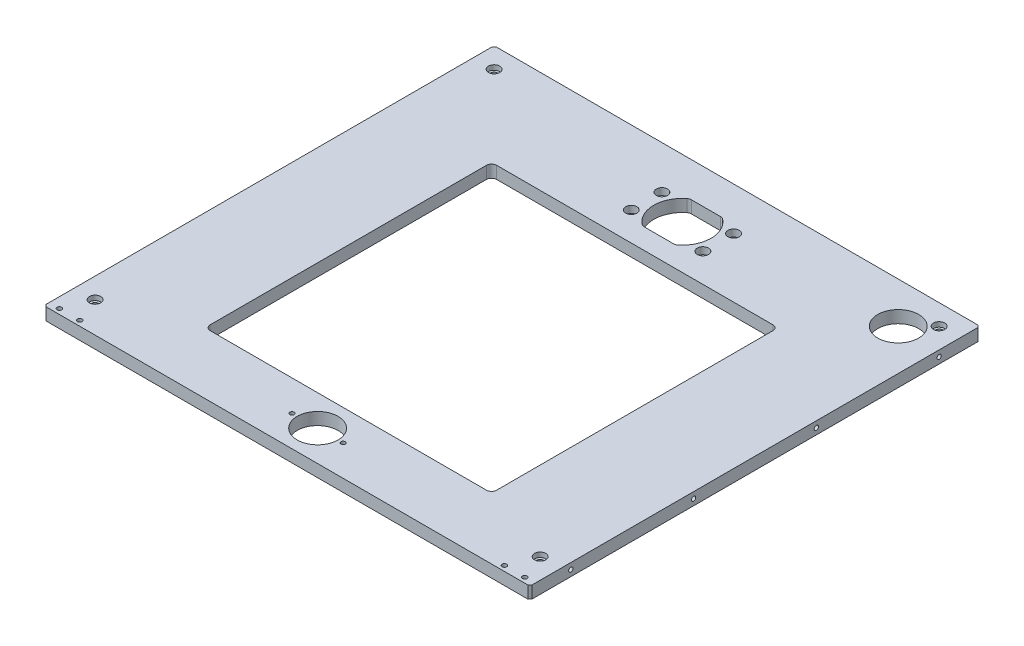
from build123d import *

# Parameters (mm, degrees)
SKETCH1_W                                       = 475
SKETCH1_H                                       = 440
BOSS_EXTRUDE1_DEPTH                             = 12
SKETCH3_R                                       = 20
CUT_EXTRUDE2_DEPTH                              = 324.960259909
HEX_SOCKET_BUTTON_HEAD_SCREW_HOLE_1_D           = 6.6
HEX_SOCKET_BUTTON_HEAD_SCREW_HOLE_1_CBORE_D     = 11
HEX_SOCKET_BUTTON_HEAD_SCREW_HOLE_1_CBORE_DEPTH = 4.7
CHAMFER1_SIZE                                   = 2
CUT_EXTRUDE4_REACH                              = 325.96
HEX_SOCKET_CAP_SCREW_HOLE_TYPE_1_D              = 6.6
HEX_SOCKET_CAP_SCREW_HOLE_TYPE_1_CBORE_D        = 11
HEX_SOCKET_CAP_SCREW_HOLE_TYPE_1_CBORE_DEPTH    = 6.8
FILLET1_R                                       = 5
M5_TAPPED_HOLE1_D                               = 4.2
M5_TAPPED_HOLE2_AT_2_COUNT                      = 2
M5_TAPPED_HOLE2_AT_2_PITCH                      = 120
M5_TAPPED_HOLE2_AT_3_COUNT                      = 2
M5_TAPPED_HOLE2_AT_3_PITCH                      = 240
M5_TAPPED_HOLE2_AT_4_COUNT                      = 2
M5_TAPPED_HOLE2_AT_4_PITCH                      = 360
M5_TAPPED_HOLE3_D                               = 4.2
M5_TAPPED_HOLE3_DEPTH                           = 14
M5_TAPPED_HOLE3_TIP                             = 1.2618073
M4_CLEARANCE_HOLE1_D                            = 4.5
SKETCH46_W                                      = 280
SKETCH46_H                                      = 280
CUT_EXTRUDE5_DEPTH                              = 324.960259909
FILLET2_R                                       = 5
SKETCH47_R                                      = 20
CUT_EXTRUDE6_DEPTH                              = 324.960259909


with BuildPart() as part:
    # Sketch1 → Boss-Extrude1 (new body)
    with BuildSketch(Plane(origin=(0, 0, 0), x_dir=(1, 0, 0), z_dir=(0, 1, 0))):
        Rectangle(SKETCH1_W, SKETCH1_H)
    extrude(amount=BOSS_EXTRUDE1_DEPTH)

    # Sketch3 → Cut-Extrude2 (cut, through all)
    with BuildSketch(Plane(origin=(0, 12, 0), x_dir=(1, 0, 0), z_dir=(0, 1, 0))):
        with Locations(Location((0, -190, 0), (0, 0, 270))):
            Circle(SKETCH3_R)
    extrude(amount=-CUT_EXTRUDE2_DEPTH, mode=Mode.SUBTRACT)

    # Hex socket button head screw hole 1 (through all)
    with Locations(Plane(origin=(0, 12, 0), x_dir=(1, 0, 0), z_dir=(0, 1, 0))):
        with Locations((217.5, 200), (217.5, -190), (-217.5, -190), (-217.5, 200)):
            CounterBoreHole(HEX_SOCKET_BUTTON_HEAD_SCREW_HOLE_1_D / 2, HEX_SOCKET_BUTTON_HEAD_SCREW_HOLE_1_CBORE_D / 2, HEX_SOCKET_BUTTON_HEAD_SCREW_HOLE_1_CBORE_DEPTH)

    # Chamfer1
    chamfer1_edges = [part.edges().sort_by_distance(p)[0] for p in [
        (237.5, 6, 220),
        (-237.5, 6, 220),
        (-237.5, 6, -220),
        (237.5, 6, -220),
    ]]
    chamfer(chamfer1_edges, length=CHAMFER1_SIZE)

    # Sketch33 → Cut-Extrude4 (cut, up to next)
    with BuildSketch(Plane(origin=(0, 12, 0), x_dir=(1, 0, 0), z_dir=(0, 1, 0)), mode=Mode.PRIVATE) as cut_extrude4_sk1:
        with BuildLine():
            Line((-12.388330441, 186), (19.549108404, 186))
            ThreePointArc((19.549108404, 186), (31.580388981, 163), (19.549108404, 140))
            Line((19.549108404, 140), (-12.388330441, 140))
            ThreePointArc((-12.388330441, 140), (-24.419611019, 163), (-12.388330441, 186))
        make_face()
    cut_extrude4_tool1 = extrude(cut_extrude4_sk1.sketch, amount=-CUT_EXTRUDE4_REACH, mode=Mode.PRIVATE) & part.part
    add(cut_extrude4_tool1.solids().sort_by_distance((3.580389, 12, -163))[0], mode=Mode.SUBTRACT)

    # Hex socket cap screw hole type 1 (through all)
    with Locations(Plane(origin=(0, 12, 0), x_dir=(1, 0, 0), z_dir=(0, 1, 0))):
        with Locations((38.580388981, 148), (38.580388981, 178), (-31.419611019, 148), (-31.419611019, 178)):
            CounterBoreHole(HEX_SOCKET_CAP_SCREW_HOLE_TYPE_1_D / 2, HEX_SOCKET_CAP_SCREW_HOLE_TYPE_1_CBORE_D / 2, HEX_SOCKET_CAP_SCREW_HOLE_TYPE_1_CBORE_DEPTH)

    # Fillet1
    fillet1_edges = [part.edges().sort_by_distance(p)[0] for p in [
        (19.549108404, 6, -186),
        (19.549108404, 6, -140),
        (-12.388330441, 6, -140),
        (-12.388330441, 6, -186),
    ]]
    fillet(fillet1_edges, radius=FILLET1_R)

    # M5 Tapped Hole1 (through all)
    with Locations(Plane(origin=(0, 12, 0), x_dir=(1, 0, 0), z_dir=(0, 1, 0))):
        with Locations((-25, -190), (25, -190)):
            Hole(M5_TAPPED_HOLE1_D / 2)

    # Sketch39 → M5 Tapped Hole2 (revolve, cut)
    with BuildSketch(Plane(origin=(-237.5, 6, -180), x_dir=(0, 0, 1), z_dir=(0, 1, 0))):
        Polygon((0, 0), (0, 15.2618073), (2.1, 14), (2.1, 0), align=None)
    m5_tapped_hole2 = revolve(axis=Axis((-243.85, 6, -180), (1, 0, 0)), mode=Mode.SUBTRACT)

    # M5 Tapped Hole2 at 2: M5 Tapped Hole2 ×2
    with Locations(*[(0, 0, i * M5_TAPPED_HOLE2_AT_2_PITCH) for i in range(1, M5_TAPPED_HOLE2_AT_2_COUNT)]):
        add(m5_tapped_hole2, mode=Mode.SUBTRACT)

    # M5 Tapped Hole2 at 3: M5 Tapped Hole2 ×2
    with Locations(*[(0, 0, i * M5_TAPPED_HOLE2_AT_3_PITCH) for i in range(1, M5_TAPPED_HOLE2_AT_3_COUNT)]):
        add(m5_tapped_hole2, mode=Mode.SUBTRACT)

    # M5 Tapped Hole2 at 4: M5 Tapped Hole2 ×2
    with Locations(*[(0, 0, i * M5_TAPPED_HOLE2_AT_4_PITCH) for i in range(1, M5_TAPPED_HOLE2_AT_4_COUNT)]):
        add(m5_tapped_hole2, mode=Mode.SUBTRACT)

    # Mirror1: M5 Tapped Hole2 across plane
    add(m5_tapped_hole2.mirror(Plane(origin=(0, 0, 0), x_dir=(0, 0, 1), z_dir=(1, 0, 0))), mode=Mode.SUBTRACT)

    # Mirror1 copy 1 sketch → Mirror1 copy 1 (revolve, cut)
    with BuildSketch(Plane(origin=(237.5, 6, -60), x_dir=(0, 0, 1), z_dir=(0, 1, 0))):
        Polygon((0, 0), (0, -15.2618073), (2.1, -14), (2.1, 0), align=None)
    revolve(axis=Axis((243.85, 6, -60), (1, 0, 0)), mode=Mode.SUBTRACT)

    # Mirror1 copy 2 sketch → Mirror1 copy 2 (revolve, cut)
    with BuildSketch(Plane(origin=(237.5, 6, 60), x_dir=(0, 0, 1), z_dir=(0, 1, 0))):
        Polygon((0, 0), (0, -15.2618073), (2.1, -14), (2.1, 0), align=None)
    revolve(axis=Axis((243.85, 6, 60), (1, 0, 0)), mode=Mode.SUBTRACT)

    # Mirror1 copy 3 sketch → Mirror1 copy 3 (revolve, cut)
    with BuildSketch(Plane(origin=(237.5, 6, 180), x_dir=(0, 0, 1), z_dir=(0, 1, 0))):
        Polygon((0, 0), (0, -15.2618073), (2.1, -14), (2.1, 0), align=None)
    revolve(axis=Axis((243.85, 6, 180), (1, 0, 0)), mode=Mode.SUBTRACT)

    # M5 Tapped Hole3
    with Locations(Plane(origin=(0, 0, -220), x_dir=(-1, 0, 0), z_dir=(0, 0, -1))):
        with Locations((-195, 6), (-65, 6), (65, 6), (195, 6)):
            Hole(M5_TAPPED_HOLE3_D / 2, depth=M5_TAPPED_HOLE3_DEPTH)
            with Locations((0, 0, -(M5_TAPPED_HOLE3_DEPTH + M5_TAPPED_HOLE3_TIP / 2))):  # 118° drill point
                Cone(0, M5_TAPPED_HOLE3_D / 2, M5_TAPPED_HOLE3_TIP, mode=Mode.SUBTRACT)

    # M4 Clearance Hole1 (through all)
    with Locations(Plane(origin=(0, 12, 0), x_dir=(1, 0, 0), z_dir=(0, 1, 0))):
        with Locations((-227.5, -215), (-207.5, -215), (207.5, -215), (227.5, -215)):
            Hole(M4_CLEARANCE_HOLE1_D / 2)

    # Sketch46 → Cut-Extrude5 (cut, through all)
    with BuildSketch(Plane(origin=(0, 12, 0), x_dir=(1, 0, 0), z_dir=(0, 1, 0))):
        with Locations((0, -20)):
            Rectangle(SKETCH46_W, SKETCH46_H)
    extrude(amount=-CUT_EXTRUDE5_DEPTH, mode=Mode.SUBTRACT)

    # Fillet2
    fillet2_edges = [part.edges().sort_by_distance(p)[0] for p in [
        (-140, 6, 160),
        (-140, 6, -120),
        (140, 6, -120),
        (140, 6, 160),
    ]]
    fillet(fillet2_edges, radius=FILLET2_R)

    # Sketch47 → Cut-Extrude6 (cut, through all)
    with BuildSketch(Plane(origin=(0, 12, 0), x_dir=(1, 0, 0), z_dir=(0, 1, 0))):
        with Locations(Location((197.5, 180, 0), (0, 0, 270))):
            Circle(SKETCH47_R)
    extrude(amount=-CUT_EXTRUDE6_DEPTH, mode=Mode.SUBTRACT)


solid = part.part
